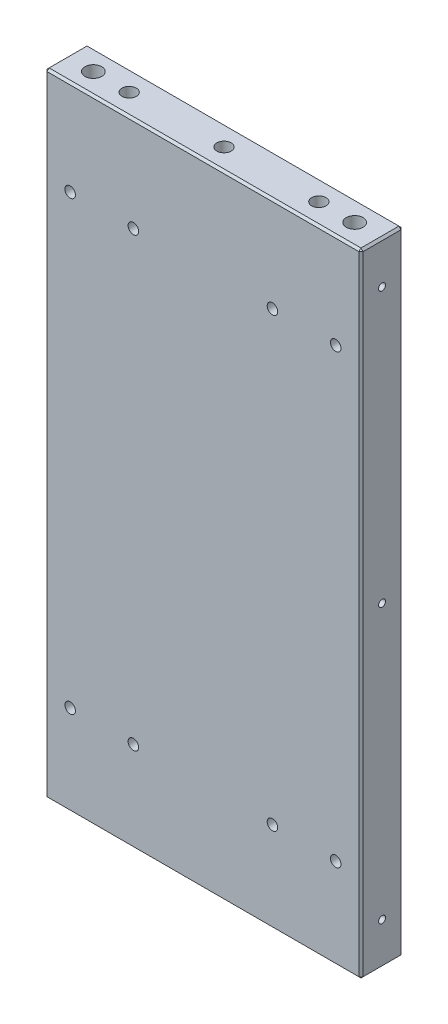
SolidWorks part; units mm, degrees
material "6061铝"
ref_plane "前视基准面" through (0, 0, 0) normal (0, 0, 1) x (1, 0, 0)
ref_plane "上视基准面" through (0, 0, 0) normal (0, 1, 0) x (1, 0, 0)
ref_plane "右视基准面" through (0, 0, 0) normal (1, 0, 0) x (0, 0, -1)
sketch "草图1" plane through (0, 0, 0) normal (0, 0, 1) x (1, 0, 0)
  line L1 (-75, 150) -> (75, 150)
  line L2 (-75, 150) -> (-75, -150)
  line L3 (-75, -150) -> (75, -150)
  line L4 (75, 150) -> (75, -150)
  line L5 (-75, 150) -> (75, -150) construction
  line L6 (-75, -150) -> (75, 150) construction
  point P0 (0, 0)
  dimension "D1" = 300
  dimension "D2" = 150
extrude "凸台-拉伸1" add sketch "草图1" along normal mid plane 20
chamfer "倒角1" distance 1 angle 45 12 edges at (0, -150, 10) (0, -150, -10) (-75, 0, 10) (-75, -150, 0) (-75, 0, -10) (0, 150, 10) (-75, 150, 0) (0, 150, -10) (75, -150, 0) (75, 0, 10) (75, 150, 0) (75, 0, -10)
hole_wizard "M8 螺纹孔1" positions "草图3" profile "草图2" tap size "M8" standard "GB"
sketch "草图3" plane through (0, 150, 0) normal (0, 1, 0) x (1, 0, 0)
  point P0 (-45, 0)
  point P5 (45, 0)
  point P9 (0, 0)
  dimension "D1" = 45
  dimension "D2" = 45
sketch "草图2" plane through (-45, 150, 0) normal (1, 0, 0) x (0, 0, 1)
  line L0 (0, 0) -> (0, 23.2929)
  line L1 (0, 23.2929) -> (3.4, 21.25)
  line L2 (3.4, 21.25) -> (3.4, 0)
  line L5 (3.4, 0) -> (0, 0)
  line L10 (0, 23.2929) -> (-3.4, 21.25) construction
  line L11 (0, -6.35) -> (0, 107.95) construction
  dimension "螺纹孔钻头直径" = 6.8
  dimension "螺纹孔钻头深度" = 21.25
  dimension "导头角度" = 118
cosmetic thread "孔螺蚊线1" parameters "D1"=15, "D2"=8
cosmetic thread "孔螺蚊线3" parameters "D1"=15, "D2"=8
cosmetic thread "孔螺蚊线44" parameters "D1"=15, "D2"=8
hole_wizard "M4 螺纹孔1" positions "草图11" profile "草图10" tap size "M4" standard "GB"
sketch "草图11" plane through (-75, 0, 0) normal (-1, 0, 0) x (0, 0, 1)
  line L1 (0, 130) -> (0, 0) construction
  line L2 (0, 0) -> (0, -130) construction
  line L5 (9, -150) -> (-9, -150) construction
  line L6 (-10, -149) -> (-10, 149) construction
  point P0 (0, -130)
  point P2 (0, 0)
  point P4 (0, 130)
  dimension "D1" = 20
  dimension "D2" = 130
  dimension "D3" = 10
sketch "草图10" plane through (-75, -130, 0) normal (0, 1, 0) x (0, 0, 1)
  line L0 (0, 0) -> (0, 12.4914)
  line L1 (0, 12.4914) -> (1.65, 11.5)
  line L2 (1.65, 11.5) -> (1.65, 0)
  line L5 (1.65, 0) -> (0, 0)
  line L10 (0, 12.4914) -> (-1.65, 11.5) construction
  line L11 (0, -6.35) -> (0, 107.95) construction
  dimension "螺纹孔钻头直径" = 3.3
  dimension "螺纹孔钻头深度" = 11.5
  dimension "导头角度" = 118
cosmetic thread "孔螺蚊线13" parameters "D1"=8, "D2"=4
cosmetic thread "孔螺蚊线14" parameters "D1"=8, "D2"=4
cosmetic thread "孔螺蚊线35" parameters "D1"=8, "D2"=4
mirror "镜向1" about plane through (0, 0, 0) normal (1, 0, 0) of "M4 螺纹孔1"
hole_wizard "大小mm 暗销孔1" positions "草图14" profile "草图16" hole size "Ø8.0" standard "GB"
sketch "草图14" plane through (0, 150, 0) normal (0, 1, 0) x (1, 0, 0)
  line L0 (0, 0) -> (0, 32.0222) construction
  point P0 (-62, 0)
  point P2 (62, 0)
  dimension "D1" = 124
sketch "草图16" plane through (-62, 150, 0) normal (1, 0, 0) x (0, 0, 1)
  line L0 (0, 0) -> (0, 17.4034)
  line L1 (0, 17.4034) -> (4, 15)
  line L2 (4, 15) -> (4, 0)
  line L5 (4, 0) -> (0, 0)
  line L10 (0, 17.4034) -> (-4, 15) construction
  line L11 (0, -6.35) -> (0, 107.95) construction
  dimension "孔直径" = 8
  dimension "孔深度" = 15
  dimension "导头角度" = 118
hole_wizard "M6 螺纹孔3" positions "草图17" profile "草图18" tap size "M6" standard "GB" end condition through all
sketch "草图17" plane through (0, 0, -10) normal (0, 0, -1) x (-1, 0, 0)
  point P0 (-33, 105)
  point P3 (-63, 105)
  point P6 (63, 105)
  point P9 (33, 105)
sketch "草图18" plane through (33, 105, -10) normal (1, 0, 0) x (0, 1, 0)
  line L0 (0, 0) -> (0, 20)
  line L1 (0, 20) -> (2.5, 20)
  line L2 (2.5, 20) -> (2.5, 0)
  line L5 (2.5, 0) -> (0, 0)
  line L11 (0, -6.35) -> (0, 107.95) construction
  dimension "通孔螺纹孔钻头直径" = 5
  dimension "通孔螺纹孔钻头深度" = 20
cosmetic thread "孔螺蚊线36" parameters "D2"=6
cosmetic thread "孔螺蚊线37" parameters "D2"=6
cosmetic thread "孔螺蚊线38" parameters "D2"=6
cosmetic thread "孔螺蚊线39" parameters "D2"=6
hole_wizard "M6 螺纹孔4" positions "草图19" profile "草图21" tap size "M6" standard "GB" end condition through all
sketch "草图19" plane through (0, 0, 10) normal (0, 0, 1) x (1, 0, 0)
  point P0 (-33, -107)
  point P3 (-63, -107)
  point P6 (33, -107)
  point P9 (63, -107)
cosmetic thread "孔螺蚊线40" parameters "D2"=6
cosmetic thread "孔螺蚊线41" parameters "D2"=6
cosmetic thread "孔螺蚊线42" parameters "D2"=6
cosmetic thread "孔螺蚊线43" parameters "D2"=6
sketch "草图21" plane through (-33, -107, 10) normal (1, 0, 0) x (0, -1, 0)
  line L0 (0, 0) -> (0, 20)
  line L1 (0, 20) -> (2.5, 20)
  line L2 (2.5, 20) -> (2.5, 0)
  line L5 (2.5, 0) -> (0, 0)
  line L11 (0, -6.35) -> (0, 107.95) construction
  dimension "通孔螺纹孔钻头直径" = 5
  dimension "通孔螺纹孔钻头深度" = 20
mirror "镜向2" about plane through (0, 0, 0) normal (0, 1, 0) of "大小mm 暗销孔1", "M8 螺纹孔1"
